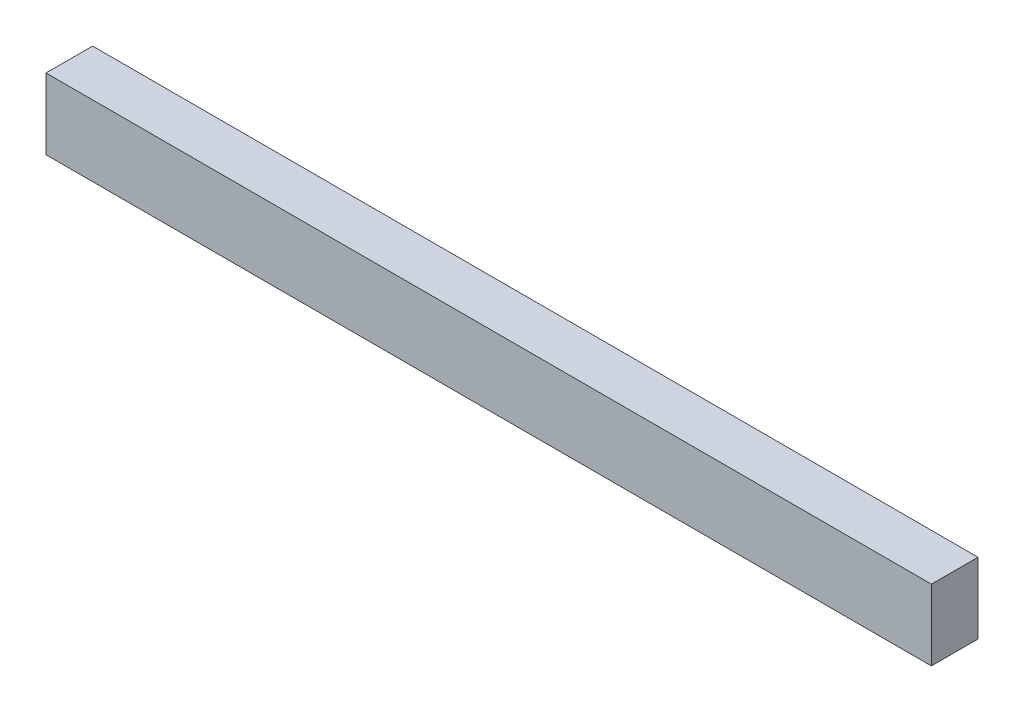
from build123d import *

# Parameters (mm, degrees)
SKETCH1_W           = 475
SKETCH1_H           = 38
BOSS_EXTRUDE1_DEPTH = 25


with BuildPart() as part:
    # Sketch1 → Boss-Extrude1 (new body)
    with BuildSketch(Plane.XY):
        Rectangle(SKETCH1_W, SKETCH1_H)
    extrude(amount=BOSS_EXTRUDE1_DEPTH)


solid = part.part
